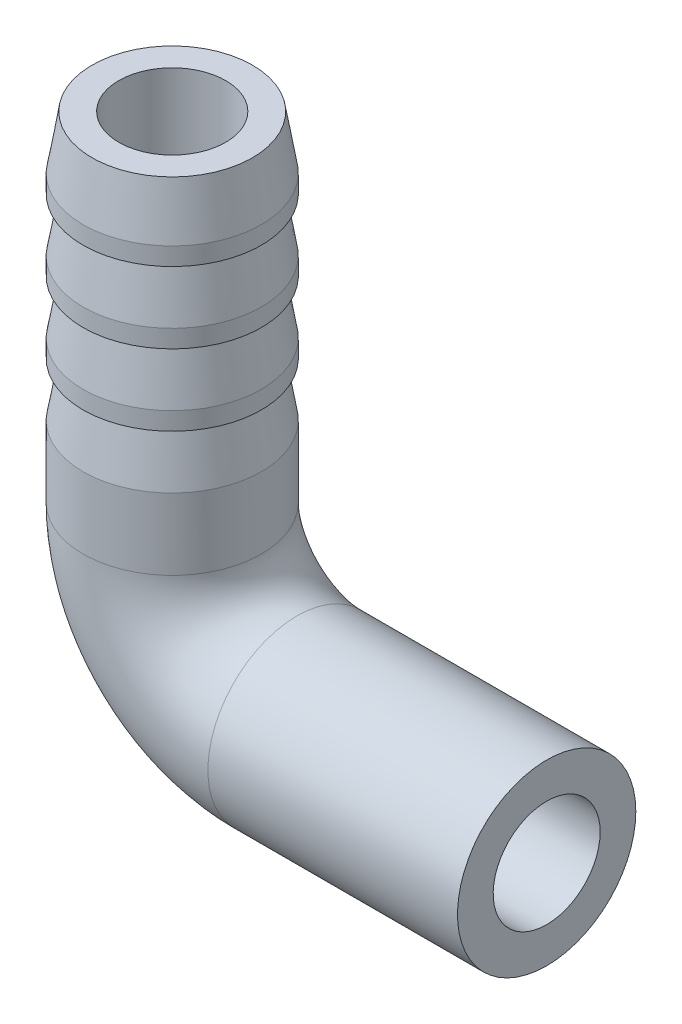
SolidWorks part; units mm, degrees
ref_plane "前视基准面" through (0, 0, 0) normal (0, 0, 1) x (1, 0, 0)
ref_plane "上视基准面" through (0, 0, 0) normal (0, 1, 0) x (1, 0, 0)
ref_plane "右视基准面" through (0, 0, 0) normal (1, 0, 0) x (0, 0, -1)
sketch "草图1" plane through (0, 0, 0) normal (0, 0, 1) x (1, 0, 0)
  line L0 (0, -266.5887) -> (0, 13062.8486) construction
  line L1 (-5, 4) -> (-4.5, 7)
  line L2 (0, 0) -> (-5, 0)
  line L3 (0, 0) -> (0, 19)
  line L5 (-5, 0) -> (-5, 4)
  line L6 (-5, 8) -> (-4.5, 11)
  line L7 (-5, 7) -> (-4.5, 7)
  line L8 (-5, 7) -> (-5, 8)
  line L11 (-4.5, -988.826) -> (-4.5, 49011.174) construction
  line L12 (-5, 11) -> (-4.5, 11)
  line L13 (-5, 11) -> (-5, 12)
  line L16 (-5, 12) -> (-4.5, 15)
  line L17 (-5, 15) -> (-4.5, 15)
  line L18 (-5, 15) -> (-5, 16)
  line L19 (-5, 16) -> (-4.5, 19)
  line L20 (-4.5, 19) -> (0, 19)
  dimension "D1" = 5
  dimension "D2" = 19
  dimension "D3" = 1
  dimension "D4" = 3
  dimension "D5" = 4.5
  dimension "D6" = 1
  dimension "D7" = 3
  dimension "D8" = 3
  dimension "D9" = 1
  dimension "D10" = 3
revolve "旋转1" add sketch "草图1" angle 360 about L3
sketch "草图2" plane through (0, 0, 0) normal (0, -1, 0) x (1, 0, 0)
  line L0 (-1000, 0) -> (49000, 0) construction
  line L1 (8.0829, 0) -> (4.0415, 7)
  line L2 (4.0415, 7) -> (-4.0415, 7)
  line L3 (-4.0415, 7) -> (-8.0829, 0)
  line L4 (-8.0829, 0) -> (-4.0415, -7)
  line L5 (-4.0415, -7) -> (4.0415, -7)
  line L6 (4.0415, -7) -> (8.0829, 0)
  circle A0 centre (0, 0) radius 7 construction
  dimension "D1" = 14
extrude "凸台-拉伸1" [suppressed] add sketch "草图2" along normal blind 4
sketch "草图4" plane through (0, 19, 0) normal (0, 1, 0) x (1, 0, 0)
  circle A0 centre (0, 0) radius 3
  dimension "D1" = 6
extrude "切除-拉伸1" cut sketch "草图4" against normal up to next
sketch "草图5" plane through (0, 0, 0) normal (0, 0, 1) x (1, 0, 0)
  line L0 (21, -7) -> (7, -7)
  line L1 (0, 0) -> (0, 21.7376) construction
  line L2 (-5, 4) -> (-5, 0) construction
  arc A0 (7, -7) -> (0, 0) centre (7, 0) cw
  dimension "D2" = 7
  dimension "D1" = 26
sketch "草图6" plane through (0, 0, 0) normal (0, -1, 0) x (1, 0, 0)
  circle A0 centre (0, 0) radius 5 construction
  circle A1 centre (0, 0) radius 3 construction
  circle A2 centre (0, 0) radius 5
  circle A3 centre (0, 0) radius 3
sweep "扫描1" add profiles "草图6" path "草图5"
